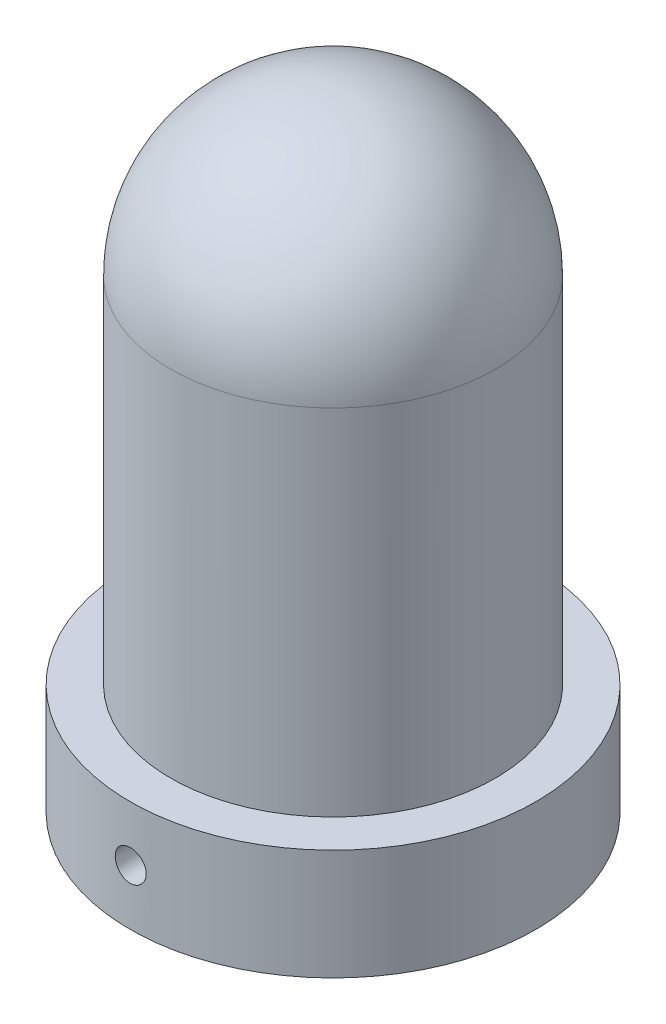
SolidWorks part; units mm, degrees
ref_plane "Front Plane" through (0, 0, 0) normal (0, 0, 1) x (1, 0, 0)
ref_plane "Top Plane" through (0, 0, 0) normal (0, 1, 0) x (1, 0, 0)
ref_plane "Right Plane" through (0, 0, 0) normal (1, 0, 0) x (0, 0, -1)
sketch "Sketch1" plane through (0, 0, 0) normal (0, 0, 1) x (1, 0, 0)
  line L0 (0, 0) -> (0, 85) construction
  line L1 (-22, 63) -> (-22, 15)
  line L2 (-22, 15) -> (-27.5, 15)
  line L3 (-27.5, 15) -> (-27.5, 0)
  line L4 (-27.5, 0) -> (-17.5, 0)
  line L5 (0, 0) -> (0, 85) construction
  line L6 (-17, 63) -> (-17, 20)
  line L7 (-17, 20) -> (-17.5, 20)
  line L8 (-17.5, 20) -> (-17.5, 0)
  line L9 (0, 85) -> (0, 80)
  line L10 (-27.5, 0) -> (0, 0) construction
  line L11 (-5, 5) -> (-5, 79.2481) construction
  line L12 (-22.5, 5) -> (-5, 5) construction
  line L13 (-22.5, 10) -> (-22.5, 5) construction
  line L14 (-17, 10) -> (-22.5, 10) construction
  line L15 (-17, 63) -> (-17, 10) construction
  arc A0 (0, 85) -> (-22, 63) centre (0, 63) ccw
  arc A1 (0, 80) -> (-17, 63) centre (0, 63) ccw
  arc A2 (-5, 79.2481) -> (-17, 63) centre (0, 63) ccw construction
  dimension "D2" = 22
  dimension "D1" = 15
  dimension "D3" = 27.5
  dimension "D4" = 63
  dimension "D6" = 20
  dimension "D7" = 17.5
  dimension "D5" = 5
revolve "Revolve2" add sketch "Sketch1" angle 360 about L0
sketch "Sketch3" plane through (0, 0, 0) normal (0, 0, 1) x (1, 0, 0)
  point P0 (0, 7.5)
  dimension "D1" = 7.5
hole_wizard "M5 Tapped Hole1" positions "3DSketch2" profile "Sketch4" tap size "M5" standard "Gb"
sketch3d "3DSketch2"
  point P0 (0, 7.5, 0)
  point P3 (0, 7.5, 0)
  point P5 (0, 7.5, 0)
  point P7 (-0.0022, 7.5242, 27.5)
sketch "Sketch4" plane through (-0.0022, 7.5242, 27.5) normal (0, 1, 0) x (1, 0, 0.0001)
  line L0 (0, 0) -> (0, 31.2618)
  line L1 (0, 31.2618) -> (2.1, 30)
  line L2 (2.1, 30) -> (2.1, 0)
  line L5 (2.1, 0) -> (0, 0)
  line L10 (0, 31.2618) -> (-2.1, 30) construction
  line L11 (0, -6.35) -> (0, 107.95) construction
  dimension "螺纹孔钻头直径" = 4.2
  dimension "螺纹孔钻头深度" = 30
  dimension "导头角度" = 118
cosmetic thread "CosmeticThread hole thread1" parameters "D1"=10.1265, "D2"=5
chamfer "Chamfer1" distance 2 angle 45 1 edges at (0, 0, -17.5)
